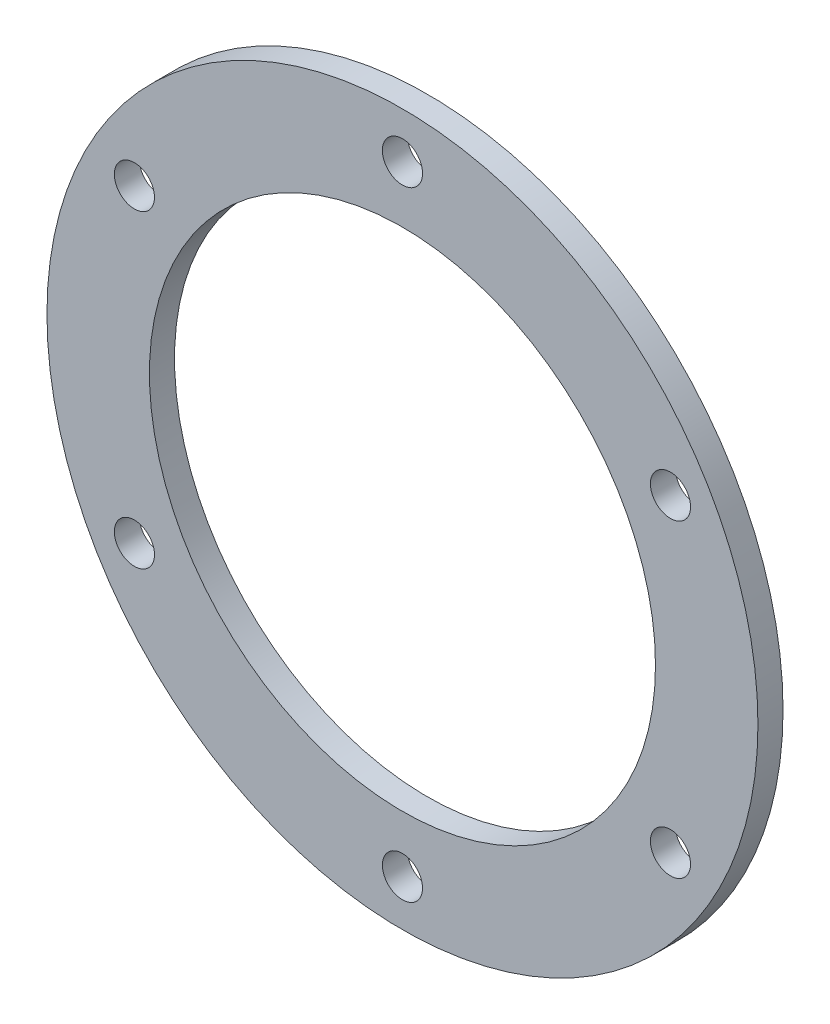
SolidWorks part; units mm, degrees
ref_plane "Front Plane" through (0, 0, 0) normal (0, 0, 1) x (1, 0, 0)
ref_plane "Top Plane" through (0, 0, 0) normal (0, 1, 0) x (1, 0, 0)
ref_plane "Right Plane" through (0, 0, 0) normal (1, 0, 0) x (0, 0, -1)
sketch "Sketch1" plane through (0, 0, 0) normal (0, 0, 1) x (1, 0, 0)
  circle A0 centre (0, 0) radius 42.5
  circle A1 centre (0, 0) radius 30.25
extrude "Boss-Extrude1" add sketch "Sketch1" along normal blind 3
sketch "Sketch2" plane through (0, 0, 3) normal (0, 0, 1) x (1, 0, 0)
  circle A1 centre (0, 37) radius 2.4
  circle A2 centre (32.0429, 18.5) radius 2.4
  circle A3 centre (32.0429, -18.5) radius 2.4
  circle A4 centre (0, -37) radius 2.4
  circle A5 centre (-32.0429, -18.5) radius 2.4
  circle A6 centre (-32.0429, 18.5) radius 2.4
  point P17 (0, 0)
  dimension "D1" = 6
extrude "Cut-Extrude1" cut sketch "Sketch2" against normal blind 3
